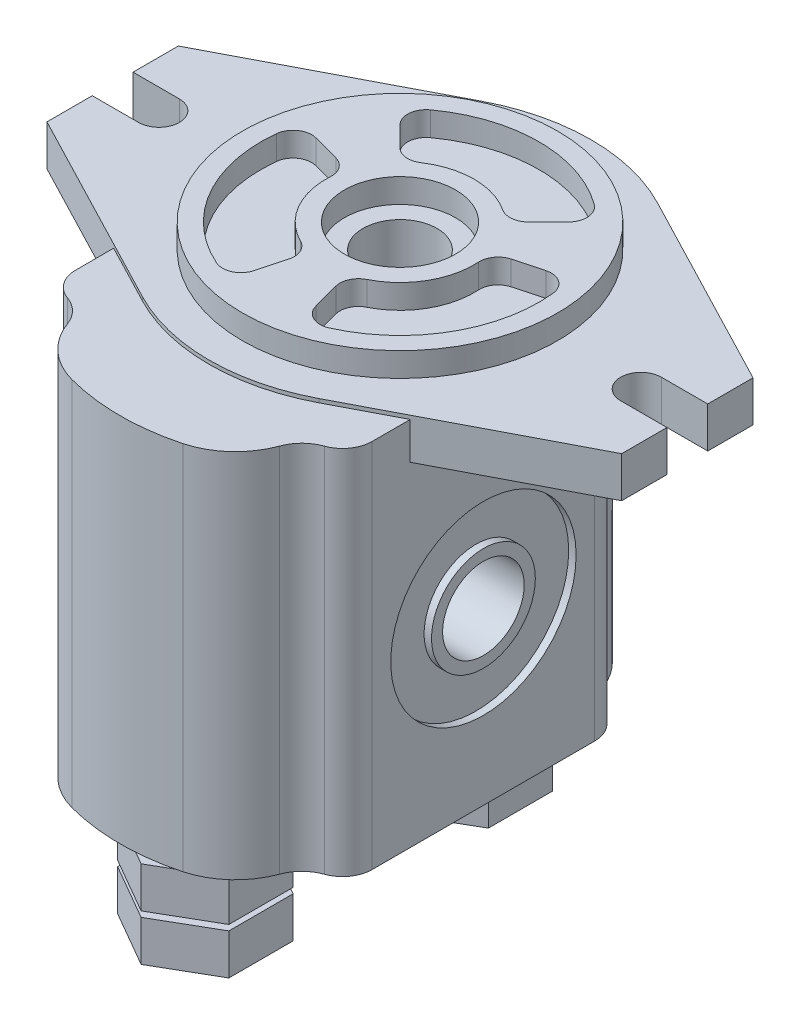
from build123d import *

# Parameters (mm, degrees)
BOSS_EXTRUDE_1_DEPTH      = 100
BOSS_EXTRUDE_2_DEPTH      = 1
BOSS_EXTRUDE_2_DEPTH_BACK = 10
SKETCH_3_R                = 42.5
SKETCH_3_R_2              = 15
BOSS_EXTRUDE_3_DEPTH      = 6.5
SKETCH_4_R                = 10
CUT_EXTRUDE_1_DEPTH       = 50
SKETCH_5_R                = 11
BOSS_EXTRUDE_4_DEPTH      = 20
SKETCH_6_R                = 25
SKETCH_6_R_2              = 14
CUT_EXTRUDE_2_DEPTH       = 2
SKETCH_7_R                = 11
CUT_EXTRUDE_3_DEPTH       = 20
BOSS_EXTRUDE_START        = -1.5
BOSS_EXTRUDE_5_DEPTH      = 11
BOSS_EXTRUDE_6_DEPTH      = 11
CUT_EXTRUDE_START         = -6
SKETCH_11_R               = 11
CUT_EXTRUDE_4_DEPTH       = 6


with BuildPart() as part:
    # Sketch 1 → Boss-Extrude 1 (new body)
    with BuildSketch(Plane(origin=(0, 0, 0), x_dir=(1, 0, 0), z_dir=(0, 1, 0))):
        with BuildLine():
            Line((-40, 30), (-40, -30))
            ThreePointArc((-40, -30), (-38.531972647, -34.618802154), (-34.666666667, -37.542472333))
            ThreePointArc((-34.666666667, -37.542472333), (-30.96133603, -39.867238912), (-28.602784398, -43.551156525))
            ThreePointArc((-28.602784398, -43.551156525), (-23.315403824, -51.462245204), (-14.970644347, -56.034630434))
            ThreePointArc((-14.970644347, -56.034630434), (0, -58), (14.970644347, -56.034630434))
            ThreePointArc((14.970644347, -56.034630434), (23.315403824, -51.462245204), (28.602784398, -43.551156525))
            ThreePointArc((28.602784398, -43.551156525), (30.96133603, -39.867238912), (34.666666667, -37.542472333))
            ThreePointArc((34.666666667, -37.542472333), (38.531972647, -34.618802154), (40, -30))
            Line((40, -30), (40, 30))
            ThreePointArc((40, 30), (38.531972647, 34.618802154), (34.666666667, 37.542472333))
            ThreePointArc((34.666666667, 37.542472333), (30.96133603, 39.867238912), (28.602784398, 43.551156525))
            ThreePointArc((28.602784398, 43.551156525), (23.315403824, 51.462245204), (14.970644347, 56.034630434))
            ThreePointArc((14.970644347, 56.034630434), (0, 58), (-14.970644347, 56.034630434))
            ThreePointArc((-14.970644347, 56.034630434), (-23.315403824, 51.462245204), (-28.602784398, 43.551156525))
            ThreePointArc((-28.602784398, 43.551156525), (-30.96133603, 39.867238912), (-34.666666667, 37.542472333))
            ThreePointArc((-34.666666667, 37.542472333), (-38.531972647, 34.618802154), (-40, 30))
        make_face()
    extrude(amount=BOSS_EXTRUDE_1_DEPTH)

    # Sketch 2 → Boss-Extrude 2 (add, two sides: drawn at the far end of the back side and taken through both)
    with BuildSketch(Plane(origin=(0, 100, 0), x_dir=(1, 0, 0), z_dir=(0, 1, 0)).offset(-BOSS_EXTRUDE_2_DEPTH_BACK)):
        with BuildLine():
            Line((-23.780053582, 63.181057909), (-77.5, 35.216223846))
            Line((-77.5, 35.216223846), (-77.5, 23))
            Line((-77.5, 23), (-65, 23))
            ThreePointArc((-65, 23), (-59.5, 17.5), (-65, 12))
            Line((-65, 12), (-77.5, 12))
            Line((-77.5, 12), (-77.5, -0.216223846))
            Line((-77.5, -0.216223846), (-23.780053582, -28.181057909))
            ThreePointArc((-23.780053582, -28.181057909), (0, -34), (23.780053582, -28.181057909))
            Line((23.780053582, -28.181057909), (77.5, -0.216223846))
            Line((77.5, -0.216223846), (77.5, 12))
            Line((77.5, 12), (65, 12))
            ThreePointArc((65, 12), (59.5, 17.5), (65, 23))
            Line((65, 23), (77.5, 23))
            Line((77.5, 23), (77.5, 35.216223846))
            Line((77.5, 35.216223846), (23.780053582, 63.181057909))
            ThreePointArc((23.780053582, 63.181057909), (0, 69), (-23.780053582, 63.181057909))
        make_face()
    extrude(amount=BOSS_EXTRUDE_2_DEPTH + BOSS_EXTRUDE_2_DEPTH_BACK)

    # Sketch 3 → Boss-Extrude 3 (add)
    with BuildSketch(Plane(origin=(0, 101, 0), x_dir=(1, 0, 0), z_dir=(0, 1, 0))):
        with Locations(Location((0, 17.5, 0), (0, 0, 90))):
            Circle(SKETCH_3_R)
        with Locations(Location((0, 17.5, 0), (0, 0, 90))):
            Circle(SKETCH_3_R_2, mode=Mode.SUBTRACT)
        with BuildLine():
            Line((-22.707377656, 40.207377656), (-17.320508076, 34.820508076))
            ThreePointArc((-17.320508076, 34.820508076), (-14.28751898, 33.381361217), (-11.027979336, 34.184833585))
            ThreePointArc((-11.027979336, 34.184833585), (0, 37.5), (11.027979336, 34.184833585))
            ThreePointArc((11.027979336, 34.184833585), (14.28751898, 33.381361217), (17.320508076, 34.820508076))
            Line((17.320508076, 34.820508076), (22.707377656, 40.207377656))
            ThreePointArc((22.707377656, 40.207377656), (24.156940055, 44.128676812), (22.121358173, 47.780282571))
            ThreePointArc((22.121358173, 47.780282571), (0, 55), (-22.121358173, 47.780282571))
            ThreePointArc((-22.121358173, 47.780282571), (-24.156940055, 44.128676812), (-22.707377656, 40.207377656))
        make_face(mode=Mode.SUBTRACT)
        with BuildLine():
            Line((31.018854731, 25.811477075), (23.660254038, 23.839745962))
            ThreePointArc((23.660254038, 23.839745962), (20.89742175, 21.932673785), (19.963479411, 18.708093465))
            ThreePointArc((19.963479411, 18.708093465), (17.320508076, 7.5), (8.935500075, -0.39292705))
            ThreePointArc((8.935500075, -0.39292705), (6.60990277, -2.814035002), (6.339745962, -6.160254038))
            Line((6.339745962, -6.160254038), (8.311477075, -13.518854731))
            ThreePointArc((8.311477075, -13.518854731), (10.982640561, -16.734862171), (15.162814854, -16.797799429))
            ThreePointArc((15.162814854, -16.797799429), (32.475952642, -1.25), (37.284173027, 21.517516858))
            ThreePointArc((37.284173027, 21.517516858), (35.139580616, 25.106185359), (31.018854731, 25.811477075))
        make_face(mode=Mode.SUBTRACT)
        with BuildLine():
            Line((-8.311477075, -13.518854731), (-6.339745962, -6.160254038))
            ThreePointArc((-6.339745962, -6.160254038), (-6.60990277, -2.814035002), (-8.935500075, -0.39292705))
            ThreePointArc((-8.935500075, -0.39292705), (-17.320508076, 7.5), (-19.963479411, 18.708093465))
            ThreePointArc((-19.963479411, 18.708093465), (-20.89742175, 21.932673785), (-23.660254038, 23.839745962))
            Line((-23.660254038, 23.839745962), (-31.018854731, 25.811477075))
            ThreePointArc((-31.018854731, 25.811477075), (-35.139580616, 25.106185359), (-37.284173027, 21.517516858))
            ThreePointArc((-37.284173027, 21.517516858), (-32.475952642, -1.25), (-15.162814854, -16.797799429))
            ThreePointArc((-15.162814854, -16.797799429), (-10.982640561, -16.734862171), (-8.311477075, -13.518854731))
        make_face(mode=Mode.SUBTRACT)
    extrude(amount=BOSS_EXTRUDE_3_DEPTH)

    # Sketch 4 → Cut-Extrude 1 (cut)
    with BuildSketch(Plane(origin=(0, 101, 0), x_dir=(1, 0, 0), z_dir=(0, 1, 0))):
        with Locations(Location((0, 17.5, 0), (0, 0, 270))):
            Circle(SKETCH_4_R)
    extrude(amount=-CUT_EXTRUDE_1_DEPTH, mode=Mode.SUBTRACT)

    # Sketch 5 → Boss-Extrude 4 (add)
    with BuildSketch(Plane.XZ):
        with Locations(Location((0, -35, 0), (0, 0, 90))):
            Circle(SKETCH_5_R)
        with Locations(Location((0, 35, 0), (0, 0, 90))):
            Circle(SKETCH_5_R)
    extrude(amount=BOSS_EXTRUDE_4_DEPTH)

    # Sketch 6 → Cut-Extrude 2 (cut)
    with BuildSketch(Plane(origin=(40, 0, 0), x_dir=(0, 0, -1), z_dir=(1, 0, 0))):
        with Locations((0, 46)):
            Circle(SKETCH_6_R)
        with Locations((0, 46)):
            Circle(SKETCH_6_R_2, mode=Mode.SUBTRACT)
    cut_extrude_2 = extrude(amount=-CUT_EXTRUDE_2_DEPTH, mode=Mode.SUBTRACT)

    # Sketch 7 → Cut-Extrude 3 (cut)
    with BuildSketch(Plane(origin=(40, 0, 0), x_dir=(0, 0, -1), z_dir=(1, 0, 0))):
        with Locations((0, 46)):
            Circle(SKETCH_7_R)
    cut_extrude_3 = extrude(amount=-CUT_EXTRUDE_3_DEPTH, mode=Mode.SUBTRACT)

    # Mirror 1: Cut-Extrude 2, Cut-Extrude 3 across plane
    add(cut_extrude_2.mirror(Plane(origin=(0, 0, 0), x_dir=(0, 0, 1), z_dir=(1, 0, 0))), mode=Mode.SUBTRACT)
    add(cut_extrude_3.mirror(Plane(origin=(0, 0, 0), x_dir=(0, 0, 1), z_dir=(1, 0, 0))), mode=Mode.SUBTRACT)

    # Sketch 9 → Boss-Extrude 5 (add)
    with BuildSketch(Plane.XZ.offset(20).offset(BOSS_EXTRUDE_START)):
        Polygon((0, -52.320508076), (15, -43.660254038), (15, -26.339745962), (0, -17.679491924), (-15, -26.339745962), (-15, -43.660254038), align=None)
        Polygon((-15, 43.660254038), (0, 52.320508076), (15, 43.660254038), (15, 26.339745962), (0, 17.679491924), (-15, 26.339745962), align=None)
    extrude(amount=-BOSS_EXTRUDE_5_DEPTH)

    # Sketch 10 → Boss-Extrude 6 (add)
    with BuildSketch(Plane.XZ.offset(20)):
        Polygon((-15, 43.660254038), (-15, 26.339745962), (0, 17.679491924), (15, 26.339745962), (15, 43.660254038), (0, 52.320508076), align=None)
        Polygon((-15, -43.660254038), (0, -52.320508076), (15, -43.660254038), (15, -26.339745962), (0, -17.679491924), (-15, -26.339745962), align=None)
    extrude(amount=BOSS_EXTRUDE_6_DEPTH)

    # Sketch 11 → Cut-Extrude 4 (cut)
    with BuildSketch(Plane.XZ.offset(31).offset(CUT_EXTRUDE_START)):
        with Locations(Location((0, -35, 0), (0, 0, 90))):
            Circle(SKETCH_11_R)
        with Locations(Location((0, 35, 0), (0, 0, 90))):
            Circle(SKETCH_11_R)
    extrude(amount=CUT_EXTRUDE_4_DEPTH, mode=Mode.SUBTRACT)


solid = part.part
